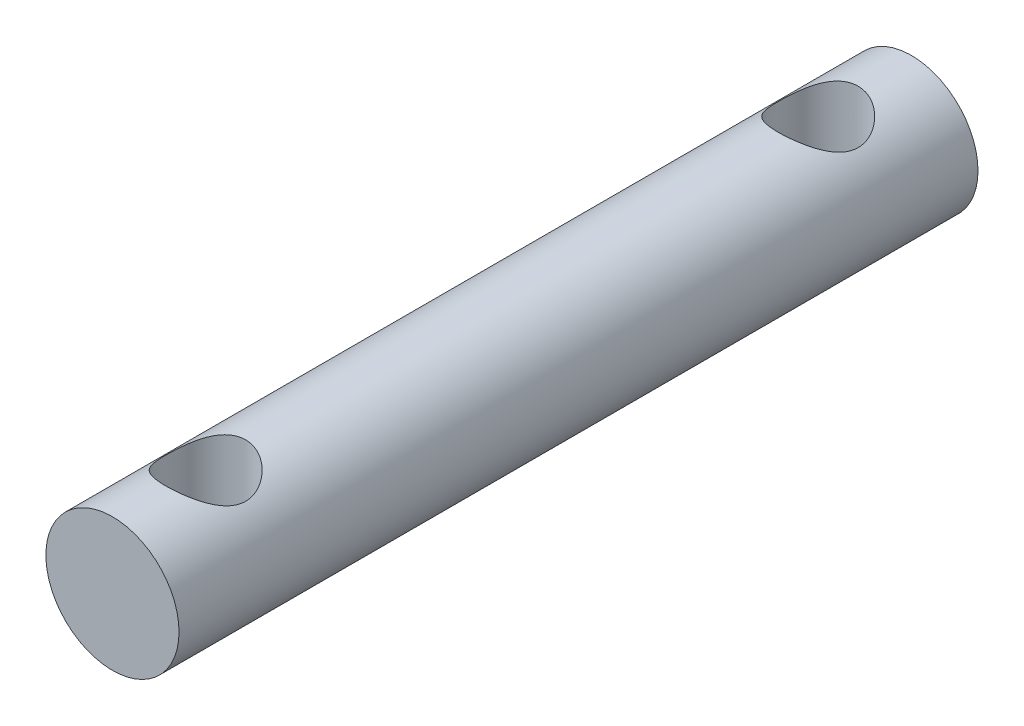
SolidWorks part; units mm, degrees
ref_plane "Front Plane" through (0, 0, 0) normal (0, 0, 1) x (1, 0, 0)
ref_plane "Top Plane" through (0, 0, 0) normal (0, 1, 0) x (1, 0, 0)
ref_plane "Right Plane" through (0, 0, 0) normal (1, 0, 0) x (0, 0, -1)
sketch "Sketch1" plane through (0, 0, 0) normal (0, 0, 1) x (1, 0, 0)
  circle A0 centre (0, 0) radius 5
  dimension "D1" = 10
extrude "Boss-Extrude1" add sketch "Sketch1" along normal blind 60
sketch "Sketch2" plane through (0, 0, 0) normal (0, 1, 0) x (1, 0, 0)
  line L2 (-5, -60) -> (5, -60) construction
  circle A0 centre (0, -7) radius 3
  circle A1 centre (0, -53) radius 3
  dimension "D1" = 6
  dimension "D2" = 40
  dimension "D4" = 7
extrude "Cut-Extrude1" cut sketch "Sketch2" against normal through all both and the other way through all
